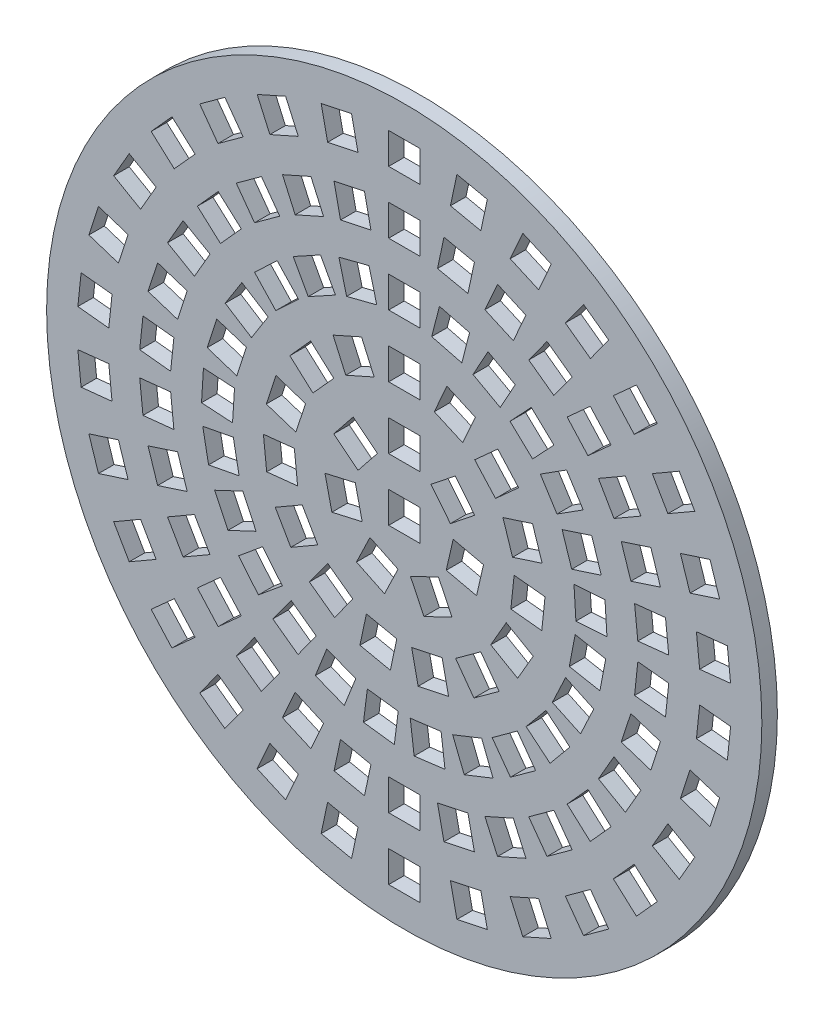
from build123d import *

# Parameters (mm, degrees)
SKETCH1_R           = 23
SKETCH1_W           = 2
SKETCH1_H           = 2
BOSS_EXTRUDE1_DEPTH = 1


with BuildPart() as part:
    # Sketch1 → Boss-Extrude1 (new body)
    with BuildSketch(Plane.XY):
        Circle(SKETCH1_R)
        Polygon((2.972174525, 18.792716105), (4.928469726, 18.376892723), (5.344293108, 20.333187925), (3.387997906, 20.749011306), align=None, mode=Mode.SUBTRACT)
        with Locations((0, 20)):
            Rectangle(SKETCH1_W, SKETCH1_H, mode=Mode.SUBTRACT)
        Polygon((6.814450761, 17.764100338), (8.641541676, 16.950627052), (9.455014962, 18.777717967), (7.627924047, 19.591191254), align=None, mode=Mode.SUBTRACT)
        Polygon((10.358902799, 15.959108145), (11.976936788, 14.783537641), (13.152507293, 16.40157163), (11.534473304, 17.577142134), align=None, mode=Mode.SUBTRACT)
        Polygon((13.450621078, 13.456626346), (14.78888229, 11.970336695), (16.275171941, 13.308597908), (14.936910729, 14.794887559), align=None, mode=Mode.SUBTRACT)
        Polygon((15.954482672, 10.366025404), (16.954482672, 8.633974596), (18.686533479, 9.633974596), (17.686533479, 11.366025404), align=None, mode=Mode.SUBTRACT)
        Polygon((17.761056815, 6.822379409), (18.379090804, 4.920266377), (20.281203837, 5.538300366), (19.663169848, 7.440413398), align=None, mode=Mode.SUBTRACT)
        Polygon((18.791387549, 2.980562697), (19.000444475, 0.991518907), (20.989488266, 1.200575833), (20.780431339, 3.189619624), align=None, mode=Mode.SUBTRACT)
        Polygon((19.000444475, -0.991518907), (18.791387549, -2.980562697), (20.780431339, -3.189619624), (20.989488266, -1.200575833), align=None, mode=Mode.SUBTRACT)
        Polygon((18.379090804, -4.920266377), (17.761056815, -6.822379409), (19.663169848, -7.440413398), (20.281203837, -5.538300366), align=None, mode=Mode.SUBTRACT)
        Polygon((16.954482672, -8.633974596), (15.954482672, -10.366025404), (17.686533479, -11.366025404), (18.686533479, -9.633974596), align=None, mode=Mode.SUBTRACT)
        Polygon((14.78888229, -11.970336695), (13.450621078, -13.456626346), (14.936910729, -14.794887559), (16.275171941, -13.308597908), align=None, mode=Mode.SUBTRACT)
        Polygon((11.976936788, -14.783537641), (10.358902799, -15.959108145), (11.534473304, -17.577142134), (13.152507293, -16.40157163), align=None, mode=Mode.SUBTRACT)
        Polygon((8.641541676, -16.950627052), (6.814450761, -17.764100338), (7.627924047, -19.591191254), (9.455014962, -18.777717967), align=None, mode=Mode.SUBTRACT)
        Polygon((4.928469726, -18.376892723), (2.972174525, -18.792716105), (3.387997906, -20.749011306), (5.344293108, -20.333187925), align=None, mode=Mode.SUBTRACT)
        with Locations((0, -20)):
            Rectangle(SKETCH1_W, SKETCH1_H, mode=Mode.SUBTRACT)
        Polygon((-2.972174525, -18.792716105), (-4.928469726, -18.376892723), (-5.344293108, -20.333187925), (-3.387997906, -20.749011306), align=None, mode=Mode.SUBTRACT)
        Polygon((-6.814450761, -17.764100338), (-8.641541676, -16.950627052), (-9.455014962, -18.777717967), (-7.627924047, -19.591191254), align=None, mode=Mode.SUBTRACT)
        Polygon((-10.358902799, -15.959108145), (-11.976936788, -14.783537641), (-13.152507293, -16.40157163), (-11.534473304, -17.577142134), align=None, mode=Mode.SUBTRACT)
        Polygon((-13.450621078, -13.456626346), (-14.78888229, -11.970336695), (-16.275171941, -13.308597908), (-14.936910729, -14.794887559), align=None, mode=Mode.SUBTRACT)
        Polygon((-15.954482672, -10.366025404), (-16.954482672, -8.633974596), (-18.686533479, -9.633974596), (-17.686533479, -11.366025404), align=None, mode=Mode.SUBTRACT)
        Polygon((-17.761056815, -6.822379409), (-18.379090804, -4.920266377), (-20.281203837, -5.538300366), (-19.663169848, -7.440413398), align=None, mode=Mode.SUBTRACT)
        Polygon((-18.791387549, -2.980562697), (-19.000444475, -0.991518907), (-20.989488266, -1.200575833), (-20.780431339, -3.189619624), align=None, mode=Mode.SUBTRACT)
        Polygon((-19.000444475, 0.991518907), (-18.791387549, 2.980562697), (-20.780431339, 3.189619624), (-20.989488266, 1.200575833), align=None, mode=Mode.SUBTRACT)
        Polygon((-18.379090804, 4.920266377), (-17.761056815, 6.822379409), (-19.663169848, 7.440413398), (-20.281203837, 5.538300366), align=None, mode=Mode.SUBTRACT)
        Polygon((-16.954482672, 8.633974596), (-15.954482672, 10.366025404), (-17.686533479, 11.366025404), (-18.686533479, 9.633974596), align=None, mode=Mode.SUBTRACT)
        Polygon((-14.78888229, 11.970336695), (-13.450621078, 13.456626346), (-14.936910729, 14.794887559), (-16.275171941, 13.308597908), align=None, mode=Mode.SUBTRACT)
        Polygon((-11.976936788, 14.783537641), (-10.358902799, 15.959108145), (-11.534473304, 17.577142134), (-13.152507293, 16.40157163), align=None, mode=Mode.SUBTRACT)
        Polygon((-8.641541676, 16.950627052), (-6.814450761, 17.764100338), (-7.627924047, 19.591191254), (-9.455014962, 18.777717967), align=None, mode=Mode.SUBTRACT)
        Polygon((-4.928469726, 18.376892723), (-2.972174525, 18.792716105), (-3.387997906, 20.749011306), (-5.344293108, 20.333187925), align=None, mode=Mode.SUBTRACT)
        Polygon((2.556351143, 16.836420903), (2.140527762, 14.880125702), (4.096822963, 14.46430232), (4.512646345, 16.420597522), align=None, mode=Mode.SUBTRACT)
        with Locations((0, 16)):
            Rectangle(SKETCH1_W, SKETCH1_H, mode=Mode.SUBTRACT)
        with Locations((0, 12)):
            Rectangle(SKETCH1_W, SKETCH1_H, mode=Mode.SUBTRACT)
        with Locations((0, 8)):
            Rectangle(SKETCH1_W, SKETCH1_H, mode=Mode.SUBTRACT)
        with Locations((0, 4)):
            Rectangle(SKETCH1_W, SKETCH1_H, mode=Mode.SUBTRACT)
        with Locations((0, 0.008481093)):
            Rectangle(SKETCH1_W, SKETCH1_H, mode=Mode.SUBTRACT)
        Polygon((6.000977475, 15.937009423), (5.187504188, 14.109918508), (7.014595104, 13.296445222), (7.82806839, 15.123536137), align=None, mode=Mode.SUBTRACT)
        Polygon((9.183332295, 14.341074157), (8.00776179, 12.723040168), (9.625795779, 11.547469663), (10.801366283, 13.165503652), align=None, mode=Mode.SUBTRACT)
        Polygon((11.964331427, 12.118365134), (10.478041776, 10.780103921), (11.816302989, 9.29381427), (13.302592639, 10.632075483), align=None, mode=Mode.SUBTRACT)
        Polygon((14.222431864, 9.366025404), (12.490381057, 8.366025404), (13.490381057, 6.633974596), (15.222431864, 7.633974596), align=None, mode=Mode.SUBTRACT)
        Polygon((15.858943783, 6.204345421), (13.95683075, 5.586311432), (14.574864739, 3.684198399), (16.476977771, 4.302232388), align=None, mode=Mode.SUBTRACT)
        Polygon((16.802343758, 2.771505771), (14.813299967, 2.562448844), (15.022356894, 0.573405054), (17.011400685, 0.78246198), align=None, mode=Mode.SUBTRACT)
        Polygon((17.011400685, -0.78246198), (15.022356894, -0.573405054), (14.813299967, -2.562448844), (16.802343758, -2.771505771), align=None, mode=Mode.SUBTRACT)
        Polygon((16.476977771, -4.302232388), (14.574864739, -3.684198399), (13.95683075, -5.586311432), (15.858943783, -6.204345421), align=None, mode=Mode.SUBTRACT)
        Polygon((15.222431864, -7.633974596), (13.490381057, -6.633974596), (12.490381057, -8.366025404), (14.222431864, -9.366025404), align=None, mode=Mode.SUBTRACT)
        Polygon((13.302592639, -10.632075483), (11.816302989, -9.29381427), (10.478041776, -10.780103921), (11.964331427, -12.118365134), align=None, mode=Mode.SUBTRACT)
        Polygon((10.801366283, -13.165503652), (9.625795779, -11.547469663), (8.00776179, -12.723040168), (9.183332295, -14.341074157), align=None, mode=Mode.SUBTRACT)
        Polygon((7.82806839, -15.123536137), (7.014595104, -13.296445222), (5.187504188, -14.109918508), (6.000977475, -15.937009423), align=None, mode=Mode.SUBTRACT)
        Polygon((4.512646345, -16.420597522), (4.096822963, -14.46430232), (2.140527762, -14.880125702), (2.556351143, -16.836420903), align=None, mode=Mode.SUBTRACT)
        with Locations((0, -16)):
            Rectangle(SKETCH1_W, SKETCH1_H, mode=Mode.SUBTRACT)
        Polygon((-2.556351143, -16.836420903), (-2.140527762, -14.880125702), (-4.096822963, -14.46430232), (-4.512646345, -16.420597522), align=None, mode=Mode.SUBTRACT)
        Polygon((-6.000977475, -15.937009423), (-5.187504188, -14.109918508), (-7.014595104, -13.296445222), (-7.82806839, -15.123536137), align=None, mode=Mode.SUBTRACT)
        Polygon((-9.183332295, -14.341074157), (-8.00776179, -12.723040168), (-9.625795779, -11.547469663), (-10.801366283, -13.165503652), align=None, mode=Mode.SUBTRACT)
        Polygon((-11.964331427, -12.118365134), (-10.478041776, -10.780103921), (-11.816302989, -9.29381427), (-13.302592639, -10.632075483), align=None, mode=Mode.SUBTRACT)
        Polygon((-14.222431864, -9.366025404), (-12.490381057, -8.366025404), (-13.490381057, -6.633974596), (-15.222431864, -7.633974596), align=None, mode=Mode.SUBTRACT)
        Polygon((-15.858943783, -6.204345421), (-13.95683075, -5.586311432), (-14.574864739, -3.684198399), (-16.476977771, -4.302232388), align=None, mode=Mode.SUBTRACT)
        Polygon((-16.802343758, -2.771505771), (-14.813299967, -2.562448844), (-15.022356894, -0.573405054), (-17.011400685, -0.78246198), align=None, mode=Mode.SUBTRACT)
        Polygon((-17.011400685, 0.78246198), (-15.022356894, 0.573405054), (-14.813299967, 2.562448844), (-16.802343758, 2.771505771), align=None, mode=Mode.SUBTRACT)
        Polygon((-16.476977771, 4.302232388), (-14.574864739, 3.684198399), (-13.95683075, 5.586311432), (-15.858943783, 6.204345421), align=None, mode=Mode.SUBTRACT)
        Polygon((-15.222431864, 7.633974596), (-13.490381057, 6.633974596), (-12.490381057, 8.366025404), (-14.222431864, 9.366025404), align=None, mode=Mode.SUBTRACT)
        Polygon((-13.302592639, 10.632075483), (-11.816302989, 9.29381427), (-10.478041776, 10.780103921), (-11.964331427, 12.118365134), align=None, mode=Mode.SUBTRACT)
        Polygon((-10.801366283, 13.165503652), (-9.625795779, 11.547469663), (-8.00776179, 12.723040168), (-9.183332295, 14.341074157), align=None, mode=Mode.SUBTRACT)
        Polygon((-7.82806839, 15.123536137), (-7.014595104, 13.296445222), (-5.187504188, 14.109918508), (-6.000977475, 15.937009423), align=None, mode=Mode.SUBTRACT)
        Polygon((-4.512646345, 16.420597522), (-4.096822963, 14.46430232), (-2.140527762, 14.880125702), (-2.556351143, 16.836420903), align=None, mode=Mode.SUBTRACT)
        Polygon((2.264385372, 12.840270982), (1.767005598, 10.90310466), (3.70417192, 10.405724885), (4.201551694, 12.342891208), align=None, mode=Mode.SUBTRACT)
        Polygon((5.386491083, 11.873740515), (4.422983735, 10.121127155), (6.175597095, 9.157619806), (7.139104443, 10.910233166), align=None, mode=Mode.SUBTRACT)
        Polygon((8.17014375, 10.161139262), (6.801049538, 8.703202008), (8.258986793, 7.334107796), (9.628081004, 8.792045051), align=None, mode=Mode.SUBTRACT)
        Polygon((10.440436237, 7.81007626), (8.751780386, 6.73842267), (9.823433976, 5.049766819), (11.512089827, 6.121420409), align=None, mode=Mode.SUBTRACT)
        Polygon((12.054717717, 4.968277443), (10.152604685, 4.350243454), (10.770638674, 2.448130422), (12.672751706, 3.066164411), align=None, mode=Mode.SUBTRACT)
        Polygon((12.91155695, 1.814303482), (10.915503493, 1.688722443), (11.041084532, -0.307331014), (13.037137989, -0.181749975), align=None, mode=Mode.SUBTRACT)
        Polygon((12.957115574, -1.453669839), (10.992541073, -1.07890721), (10.617778443, -3.043481711), (12.582352945, -3.41824434), align=None, mode=Mode.SUBTRACT)
        Polygon((12.188530974, -4.630303738), (10.378876869, -3.778745155), (9.527318286, -5.58839926), (11.33697239, -6.439957843), align=None, mode=Mode.SUBTRACT)
        Polygon((10.654096146, -7.515998624), (9.11306966, -6.241150644), (7.838221681, -7.78217713), (9.379248166, -9.05702511), align=None, mode=Mode.SUBTRACT)
        Polygon((8.450225274, -9.929435675), (7.27465477, -8.311401686), (5.656620781, -9.48697219), (6.832191285, -11.105006179), align=None, mode=Mode.SUBTRACT)
        Polygon((5.715395671, -11.718969764), (4.979146565, -9.859416792), (3.119593594, -10.595665897), (3.855842699, -12.455218869), align=None, mode=Mode.SUBTRACT)
        Polygon((2.621446738, -12.772157884), (2.370780271, -10.787928481), (0.386550868, -11.038594948), (0.637217335, -13.022824351), align=None, mode=Mode.SUBTRACT)
        Polygon((-0.637217335, -13.022824351), (-0.386550868, -11.038594948), (-2.370780271, -10.787928481), (-2.621446738, -12.772157884), align=None, mode=Mode.SUBTRACT)
        Polygon((-3.855842699, -12.455218869), (-3.119593594, -10.595665897), (-4.979146565, -9.859416792), (-5.715395671, -11.718969764), align=None, mode=Mode.SUBTRACT)
        Polygon((-6.832191285, -11.105006179), (-5.656620781, -9.48697219), (-7.27465477, -8.311401686), (-8.450225274, -9.929435675), align=None, mode=Mode.SUBTRACT)
        Polygon((-9.379248166, -9.05702511), (-7.838221681, -7.78217713), (-9.11306966, -6.241150644), (-10.654096146, -7.515998624), align=None, mode=Mode.SUBTRACT)
        Polygon((-11.33697239, -6.439957843), (-9.527318286, -5.58839926), (-10.378876869, -3.778745155), (-12.188530974, -4.630303738), align=None, mode=Mode.SUBTRACT)
        Polygon((-12.582352945, -3.41824434), (-10.617778443, -3.043481711), (-10.992541073, -1.07890721), (-12.957115574, -1.453669839), align=None, mode=Mode.SUBTRACT)
        Polygon((-13.037137989, -0.181749975), (-11.041084532, -0.307331014), (-10.915503493, 1.688722443), (-12.91155695, 1.814303482), align=None, mode=Mode.SUBTRACT)
        Polygon((-12.672751706, 3.066164411), (-10.770638674, 2.448130422), (-10.152604685, 4.350243454), (-12.054717717, 4.968277443), align=None, mode=Mode.SUBTRACT)
        Polygon((-11.512089827, 6.121420409), (-9.823433976, 5.049766819), (-8.751780386, 6.73842267), (-10.440436237, 7.81007626), align=None, mode=Mode.SUBTRACT)
        Polygon((-9.628081004, 8.792045051), (-8.258986793, 7.334107796), (-6.801049538, 8.703202008), (-8.17014375, 10.161139262), align=None, mode=Mode.SUBTRACT)
        Polygon((-7.139104443, 10.910233166), (-6.175597095, 9.157619806), (-4.422983735, 10.121127155), (-5.386491083, 11.873740515), align=None, mode=Mode.SUBTRACT)
        Polygon((-4.201551694, 12.342891208), (-3.70417192, 10.405724885), (-1.767005598, 10.90310466), (-2.264385372, 12.840270982), align=None, mode=Mode.SUBTRACT)
        Polygon((2.74708433, 8.628645762), (1.933611044, 6.801554847), (3.760701959, 5.98808156), (4.574175245, 7.815172476), align=None, mode=Mode.SUBTRACT)
        Polygon((6.019172823, 6.765320283), (4.532883172, 5.42705907), (5.871144385, 3.940769419), (7.357434036, 5.279030632), align=None, mode=Mode.SUBTRACT)
        Polygon((8.250491652, 3.732209466), (6.34837862, 3.114175477), (6.966412608, 1.212062444), (8.868525641, 1.830096433), align=None, mode=Mode.SUBTRACT)
        Polygon((9.055225522, 0.053765726), (7.066181731, 0.262822652), (6.857124804, -1.726221138), (8.846168595, -1.935278065), align=None, mode=Mode.SUBTRACT)
        Polygon((8.294228634, -3.633974596), (6.562177826, -2.633974596), (5.562177826, -4.366025404), (7.294228634, -5.366025404), align=None, mode=Mode.SUBTRACT)
        Polygon((6.099084265, -6.693367697), (4.92351376, -5.075333708), (3.305479772, -6.250904213), (4.481050276, -7.868938202), align=None, mode=Mode.SUBTRACT)
        Polygon((2.849352818, -8.595416716), (2.433529436, -6.639121514), (0.477234235, -7.054944896), (0.893057617, -9.011240097), align=None, mode=Mode.SUBTRACT)
        Polygon((-0.893057617, -9.011240097), (-0.477234235, -7.054944896), (-2.433529436, -6.639121514), (-2.849352818, -8.595416716), align=None, mode=Mode.SUBTRACT)
        Polygon((-4.481050276, -7.868938202), (-3.305479772, -6.250904213), (-4.92351376, -5.075333708), (-6.099084265, -6.693367697), align=None, mode=Mode.SUBTRACT)
        Polygon((-7.294228634, -5.366025404), (-5.562177826, -4.366025404), (-6.562177826, -2.633974596), (-8.294228634, -3.633974596), align=None, mode=Mode.SUBTRACT)
        Polygon((-8.846168595, -1.935278065), (-6.857124804, -1.726221138), (-7.066181731, 0.262822652), (-9.055225522, 0.053765726), align=None, mode=Mode.SUBTRACT)
        Polygon((-8.868525641, 1.830096433), (-6.966412608, 1.212062444), (-6.34837862, 3.114175477), (-8.250491652, 3.732209466), align=None, mode=Mode.SUBTRACT)
        Polygon((-7.357434036, 5.279030632), (-5.871144385, 3.940769419), (-4.532883172, 5.42705907), (-6.019172823, 6.765320283), align=None, mode=Mode.SUBTRACT)
        Polygon((-4.574175245, 7.815172476), (-3.760701959, 5.98808156), (-1.933611044, 6.801554847), (-2.74708433, 8.628645762), align=None, mode=Mode.SUBTRACT)
        Polygon((3.28566761, 3.899280492), (1.722004646, 2.652300888), (2.968984249, 1.088637923), (4.532647214, 2.335617527), align=None, mode=Mode.SUBTRACT)
        Polygon((5.097160495, -0.137676758), (3.147304671, 0.30736511), (2.702262803, -1.642490714), (4.652118627, -2.087532582), align=None, mode=Mode.SUBTRACT)
        Polygon((3.070387563, -4.0709606), (2.202620085, -2.269022865), (0.400682349, -3.136790343), (1.268449828, -4.938728079), align=None, mode=Mode.SUBTRACT)
        Polygon((-1.268449828, -4.938728079), (-0.400682349, -3.136790343), (-2.202620085, -2.269022865), (-3.070387563, -4.0709606), align=None, mode=Mode.SUBTRACT)
        Polygon((-4.652118627, -2.087532582), (-2.702262803, -1.642490714), (-3.147304671, 0.30736511), (-5.097160495, -0.137676758), align=None, mode=Mode.SUBTRACT)
        Polygon((-4.532647214, 2.335617527), (-2.968984249, 1.088637923), (-1.722004646, 2.652300888), (-3.28566761, 3.899280492), align=None, mode=Mode.SUBTRACT)
    extrude(amount=BOSS_EXTRUDE1_DEPTH)


solid = part.part
